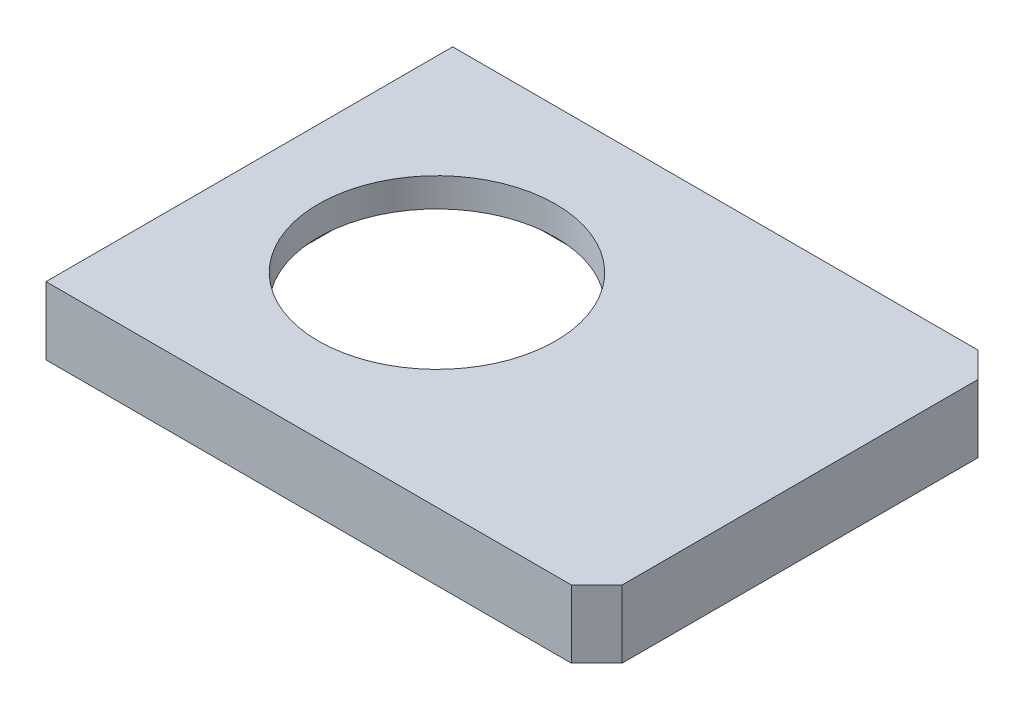
SolidWorks part; units mm, degrees
ref_plane "前视基准面" through (0, 0, 0) normal (0, 0, 1) x (1, 0, 0)
ref_plane "上视基准面" through (0, 0, 0) normal (0, 1, 0) x (1, 0, 0)
ref_plane "右视基准面" through (0, 0, 0) normal (1, 0, 0) x (0, 0, -1)
sketch "草图1" plane through (0, 0, 0) normal (0, 1, 0) x (1, 0, 0)
  line L1 (-162.5, -120) -> (162.5, -120)
  line L2 (-162.5, -120) -> (-162.5, 120)
  line L3 (-162.5, 120) -> (162.5, 120)
  line L4 (162.5, -120) -> (162.5, 120)
  line L5 (-162.5, -120) -> (162.5, 120) construction
  line L6 (-162.5, 120) -> (162.5, -120) construction
  point P0 (0, 0)
  dimension "D1" = 240
  dimension "D2" = 325
extrude "凸台-拉伸1" add sketch "草图1" along normal blind 40
sketch "草图2" plane through (0, 0, 0) normal (0, -1, 0) x (1, 0, 0)
  line L1 (40.7062, -92.5) -> (-144.2938, -92.5)
  line L2 (40.7062, -92.5) -> (40.7062, 92.5)
  line L3 (40.7062, 92.5) -> (-144.2938, 92.5)
  line L4 (-144.2938, -92.5) -> (-144.2938, 92.5)
  line L5 (40.7062, -92.5) -> (-144.2938, 92.5) construction
  line L6 (40.7062, 92.5) -> (-144.2938, -92.5) construction
  line L7 (-162.5, 120) -> (162.5, 120) construction
  line L9 (-162.5, -120) -> (-162.5, 120) construction
  point P0 (-51.7938, 0)
  dimension "D1" = 120
  dimension "D2" = 18.2062
  dimension "D3" = 185
extrude "切除-拉伸1" cut sketch "草图2" against normal blind 23
sketch "草图3" plane through (0, 23, 0) normal (0, -1, 0) x (1, 0, 0)
  line L0 (-144.2938, 92.5) -> (40.7062, -92.5) construction
  line L1 (40.7062, 92.5) -> (-144.2938, 92.5) construction
  line L2 (-144.2938, 92.5) -> (-144.2938, -92.5) construction
  line L3 (40.7062, -92.5) -> (40.7062, 92.5) construction
  circle A0 centre (-51.7938, 0) radius 70
  point P10 (-51.7938, 0)
  dimension "D1" = 140
extrude "切除-拉伸2" cut sketch "草图3" against normal through all
fillet "圆角1" radius 5 4 edges at (-144.2938, 11.5, 92.5) (40.7062, 11.5, 92.5) (40.7062, 11.5, -92.5) (-144.2938, 11.5, -92.5)
chamfer "倒角1" distance 15 angle 45 2 edges at (162.5, 20, -120) (162.5, 20, 120)
